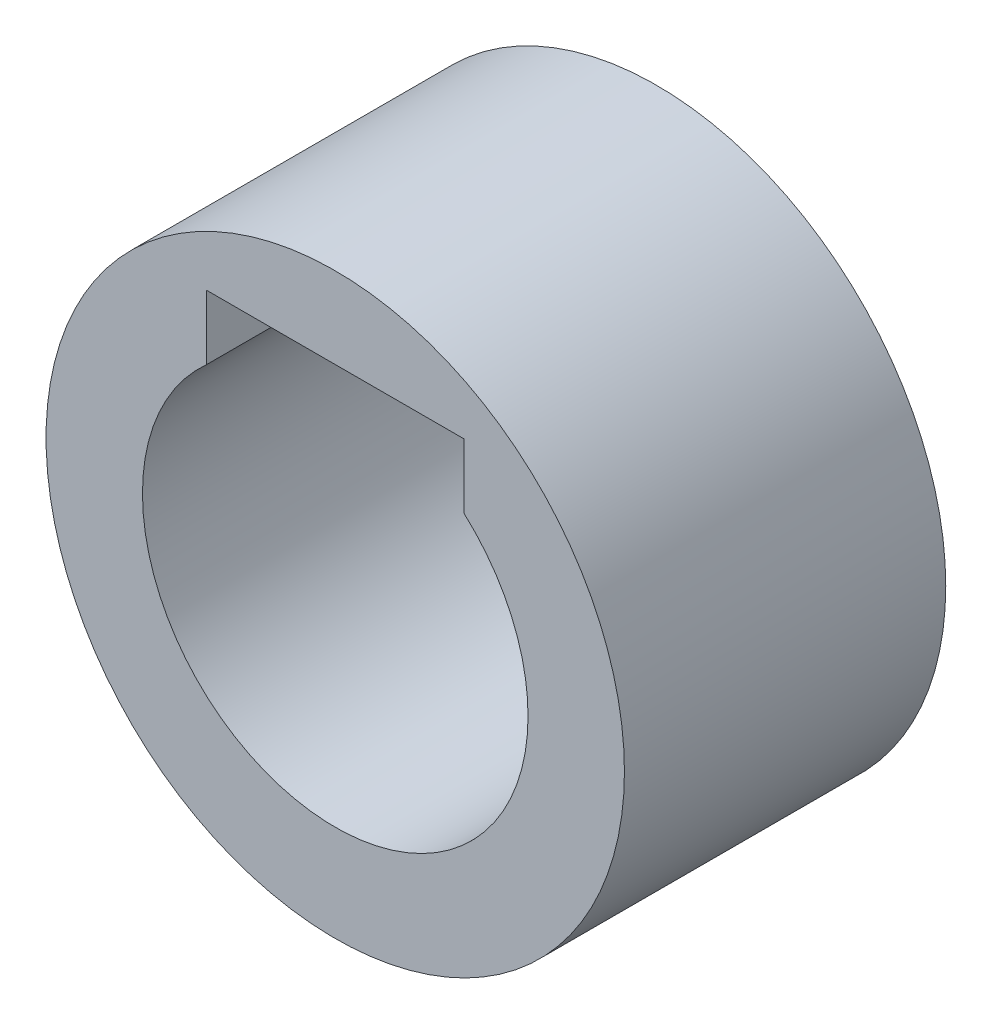
from build123d import *

# Parameters (mm, degrees)
SKETCH_1_R      = 9
EXTRUDE_1_DEPTH = 10


with BuildPart() as part:
    # 草图1 → 凸台-拉伸1 (new body)
    with BuildSketch(Plane.XY):
        with Locations((-0.274924045, -0.151737187)):
            Circle(SKETCH_1_R)
        with BuildLine():
            Line((-4.274924045, 6.320398768), (3.725075955, 6.320398768))
            Line((3.725075955, 6.320398768), (3.725075955, 4.320398768))
            ThreePointArc((3.725075955, 4.320398768), (-0.274924045, -6.151737187), (-4.274924045, 4.320398768))
            Line((-4.274924045, 4.320398768), (-4.274924045, 6.320398768))
        make_face(mode=Mode.SUBTRACT)
    extrude(amount=EXTRUDE_1_DEPTH)


solid = part.part
